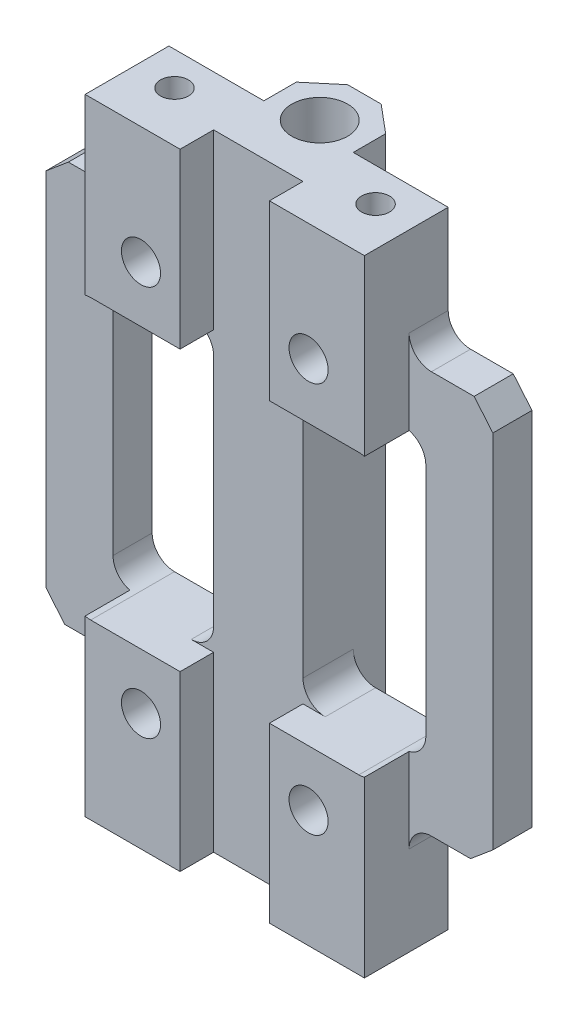
from build123d import *
from OCP.BRepFilletAPI import BRepFilletAPI_MakeChamfer

# Parameters (mm, degrees)
SKETCH1_W             = 25
SKETCH1_H             = 12.5
BOSS_EXTRUDE1_DEPTH   = 56
SKETCH3_W             = 8.5
SKETCH3_H             = 56
CUT_EXTRUDE2_DEPTH    = 5
SKETCH4_R             = 2.5
CUT_EXTRUDE3_DEPTH    = 58.717523336
SKETCH5_R             = 1.75
CUT_EXTRUDE4_DEPTH    = 58.866225037
SKETCH6_R             = 3
CUT_EXTRUDE5_DEPTH    = 3.5
CHAMFER1_SIZE         = 2.5
CHAMFER1_SIZE2        = 2.097749078
SKETCH8_W             = 7.5
SKETCH8_H             = 36
BOSS_EXTRUDE3_DEPTH   = 3.5
M3_TAPPED_HOLE1_D     = 2.5
M3_TAPPED_HOLE1_DEPTH = 7.5
M3_TAPPED_HOLE1_TIP   = 0.751075774
M3_TAPPED_HOLE2_D     = 2.5
M3_TAPPED_HOLE2_DEPTH = 7.5
M3_TAPPED_HOLE2_TIP   = 0.751075774
CHAMFER2_SIZE         = 2
CHAMFER2_SIZE2        = 1.678199262
FILLET1_R             = 2
CUT_EXTRUDE7_DEPTH    = 3
SKETCH17_W            = 10
SKETCH17_H            = 25
CUT_EXTRUDE8_DEPTH    = 10
FILLET3_R             = 2


with BuildPart() as part:
    # Sketch1 → Boss-Extrude1 (new body)
    with BuildSketch(Plane(origin=(0, 0, 0), x_dir=(1, 0, 0), z_dir=(0, 1, 0))):
        Rectangle(SKETCH1_W, SKETCH1_H)
    extrude(amount=BOSS_EXTRUDE1_DEPTH)

    # Sketch3 → Cut-Extrude2 (cut)
    with BuildSketch(Plane(origin=(0, 0, -6.25), x_dir=(-1, 0, 0), z_dir=(0, 0, -1))):
        with Locations((-8.25, 28)):
            Rectangle(SKETCH3_W, SKETCH3_H)
        with Locations((8.25, 28)):
            Rectangle(SKETCH3_W, SKETCH3_H)
    extrude(amount=-CUT_EXTRUDE2_DEPTH, mode=Mode.SUBTRACT)

    # Sketch4 → Cut-Extrude3 (cut, through all)
    with BuildSketch(Plane.XZ):
        with Locations(Location((0, -2.25, 0), (0, 0, 270))):
            Circle(SKETCH4_R)
    extrude(amount=-CUT_EXTRUDE3_DEPTH, mode=Mode.SUBTRACT)

    # Sketch5 → Cut-Extrude4 (cut, through all)
    with BuildSketch(Plane(origin=(0, 0, -1.25), x_dir=(-1, 0, 0), z_dir=(0, 0, -1))):
        with Locations((-7.5, 45.5)):
            Circle(SKETCH5_R)
        with Locations((7.5, 45.5)):
            Circle(SKETCH5_R)
        with Locations((7.5, 10.5)):
            Circle(SKETCH5_R)
        with Locations((-7.5, 10.5)):
            Circle(SKETCH5_R)
    extrude(amount=-CUT_EXTRUDE4_DEPTH, mode=Mode.SUBTRACT)

    # Sketch6 → Cut-Extrude5 (cut)
    with BuildSketch(Plane(origin=(0, 0, -1.25), x_dir=(-1, 0, 0), z_dir=(0, 0, -1))):
        with Locations((-7.5, 45.5)):
            Circle(SKETCH6_R)
        with Locations((7.5, 45.5)):
            Circle(SKETCH6_R)
        with Locations((7.5, 10.5)):
            Circle(SKETCH6_R)
        with Locations((-7.5, 10.5)):
            Circle(SKETCH6_R)
    extrude(amount=-CUT_EXTRUDE5_DEPTH, mode=Mode.SUBTRACT)

    # Chamfer1
    chamfer1_edges = [part.edges().sort_by_distance(p)[0] for p in [
        (4, 28, -6.25),
        (-4, 28, -6.25),
    ]]
    chamfer1_side = [part.faces().sort_by_distance(p)[0] for p in [
        (0, 28, -6.25),
    ]]
    chamfer(chamfer1_edges, length=CHAMFER1_SIZE, length2=CHAMFER1_SIZE2, reference=chamfer1_side[0])

    # Sketch8 → Boss-Extrude3 (add)
    with BuildSketch(Plane(origin=(0, 0, -1.25), x_dir=(-1, 0, 0), z_dir=(0, 0, -1))):
        with Locations((-16.25, 28)):
            Rectangle(SKETCH8_W, SKETCH8_H)
        with Locations((16.25, 28)):
            Rectangle(SKETCH8_W, SKETCH8_H)
    extrude(amount=-BOSS_EXTRUDE3_DEPTH)

    # M3 Tapped Hole1
    with Locations(Plane(origin=(0, 0, 0), x_dir=(-1, 0, 0), z_dir=(0, -1, 0))):
        with Locations((-9, -1.75), (9, -1.75)):
            Hole(M3_TAPPED_HOLE1_D / 2, depth=M3_TAPPED_HOLE1_DEPTH)
            with Locations((0, 0, -(M3_TAPPED_HOLE1_DEPTH + M3_TAPPED_HOLE1_TIP / 2))):  # 118° drill point
                Cone(0, M3_TAPPED_HOLE1_D / 2, M3_TAPPED_HOLE1_TIP, mode=Mode.SUBTRACT)

    # M3 Tapped Hole2
    with Locations(Plane(origin=(0, 56, 0), x_dir=(1, 0, 0), z_dir=(0, 1, 0))):
        with Locations((-9, -1.75), (9, -1.75)):
            Hole(M3_TAPPED_HOLE2_D / 2, depth=M3_TAPPED_HOLE2_DEPTH)
            with Locations((0, 0, -(M3_TAPPED_HOLE2_DEPTH + M3_TAPPED_HOLE2_TIP / 2))):  # 118° drill point
                Cone(0, M3_TAPPED_HOLE2_D / 2, M3_TAPPED_HOLE2_TIP, mode=Mode.SUBTRACT)

    # Chamfer2: one chamfer whose edges measure the first distance from different faces: ONE call of the kernel's chamfer builder (chamfer() names one face for all edges)
    chamfer2_edges_1 = [part.edges().sort_by_distance(p)[0] for p in [
        (-20, 46, 0.5),
    ]]
    chamfer2_side_1 = [part.faces().sort_by_distance(p)[0] for p in [
        (-16.25, 46, 0.5),
    ]]
    chamfer2_edges_2 = [part.edges().sort_by_distance(p)[0] for p in [
        (20, 46, 0.5),
    ]]
    chamfer2_side_2 = [part.faces().sort_by_distance(p)[0] for p in [
        (20, 28, 0.5),
    ]]
    chamfer2_edges_3 = [part.edges().sort_by_distance(p)[0] for p in [
        (20, 10, 0.5),
    ]]
    chamfer2_side_3 = [part.faces().sort_by_distance(p)[0] for p in [
        (16.25, 10, 0.5),
    ]]
    chamfer2_edges_4 = [part.edges().sort_by_distance(p)[0] for p in [
        (-20, 10, 0.5),
    ]]
    chamfer2_side_4 = [part.faces().sort_by_distance(p)[0] for p in [
        (-20, 28, 0.5),
    ]]
    chamfer2 = BRepFilletAPI_MakeChamfer(part.part.solid().wrapped)
    for e in chamfer2_edges_1:
        chamfer2.Add(CHAMFER2_SIZE, CHAMFER2_SIZE2, e.wrapped, chamfer2_side_1[0].wrapped)  # the first distance lies on this face
    for e in chamfer2_edges_2:
        chamfer2.Add(CHAMFER2_SIZE, CHAMFER2_SIZE2, e.wrapped, chamfer2_side_2[0].wrapped)  # the first distance lies on this face
    for e in chamfer2_edges_3:
        chamfer2.Add(CHAMFER2_SIZE, CHAMFER2_SIZE2, e.wrapped, chamfer2_side_3[0].wrapped)  # the first distance lies on this face
    for e in chamfer2_edges_4:
        chamfer2.Add(CHAMFER2_SIZE, CHAMFER2_SIZE2, e.wrapped, chamfer2_side_4[0].wrapped)  # the first distance lies on this face
    add(Compound.cast(chamfer2.Shape()), mode=Mode.REPLACE)

    # Fillet1
    fillet1_edges = [part.edges().sort_by_distance(p)[0] for p in [
        (-12.5, 46, 0.5),
        (12.5, 46, 0.5),
        (12.5, 10, 0.5),
        (-12.5, 10, 0.5),
    ]]
    fillet(fillet1_edges, radius=FILLET1_R)

    # Sketch16 → Cut-Extrude7 (cut)
    with BuildSketch(Plane.XY.offset(6.25)):
        Polygon((4, 40.5), (8.5, 40.5), (8.5, 15.5), (4, 15.5), (4, 0), (-4, 0), (-4, 15.5), (-8.5, 15.5), (-8.5, 40.5), (-4, 40.5), (-4, 56), (4, 56), align=None)
    extrude(amount=-CUT_EXTRUDE7_DEPTH, mode=Mode.SUBTRACT)

    # Sketch17 → Cut-Extrude8 (cut)
    with BuildSketch(Plane(origin=(0, 0, -1.25), x_dir=(-1, 0, 0), z_dir=(0, 0, -1))):
        with Locations((-9, 28)):
            Rectangle(SKETCH17_W, SKETCH17_H)
        with Locations((9, 28)):
            Rectangle(SKETCH17_W, SKETCH17_H)
    extrude(amount=-CUT_EXTRUDE8_DEPTH, mode=Mode.SUBTRACT)

    # Fillet3
    fillet3_edges = [part.edges().sort_by_distance(p)[0] for p in [
        (-4, 15.5, 1),
        (4, 15.5, 1),
        (4, 40.5, 1),
        (-14, 40.5, 0.5),
        (-14, 15.5, 0.5),
        (14, 15.5, 0.5),
        (14, 40.5, 0.5),
        (-4, 40.5, 1),
    ]]
    fillet(fillet3_edges, radius=FILLET3_R)


solid = part.part
